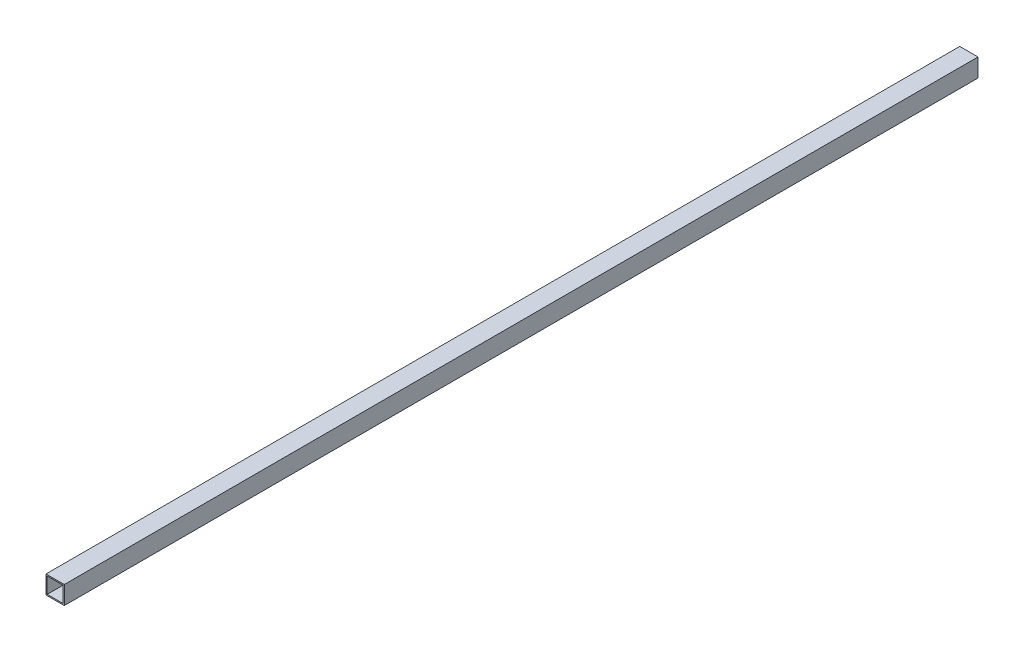
from build123d import *

# Parameters (mm, degrees)
SKETCH_1_W      = 30
SKETCH_1_H      = 30
SKETCH_1_W_2    = 26
SKETCH_1_H_2    = 26
EXTRUDE_1_DEPTH = 750


with BuildPart() as part:
    # 草图1 → 凸台-拉伸1 (new, symmetric)
    with BuildSketch(Plane.XY):
        Rectangle(SKETCH_1_W, SKETCH_1_H)
        Rectangle(SKETCH_1_W_2, SKETCH_1_H_2, mode=Mode.SUBTRACT)
    extrude(amount=EXTRUDE_1_DEPTH, both=True)


solid = part.part
